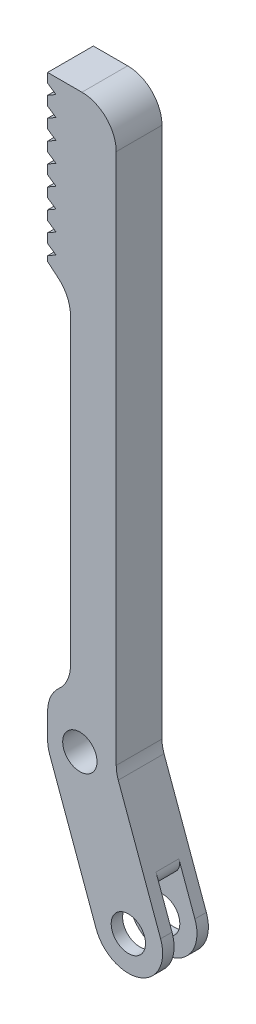
from build123d import *

# Parameters (mm, degrees)
BOSS_EXTRUDE1_DEPTH            = 20
CUT_EXTRUDE1_REACH             = 326.283
SKETCH2_W                      = 10
SKETCH2_H                      = 33.118542384
CUT_EXTRUDE2_DEPTH             = 329.583692554
F_15_0_15_DIAMETER_HOLE1_D     = 15
F_15_0_15_DIAMETER_HOLE1_DEPTH = 5
F_15_0_15_DIAMETER_HOLE2_D     = 15
F_15_0_15_DIAMETER_HOLE3_D     = 15
FILLET1_R                      = 5
FILLET2_R                      = 15
CUT_EXTRUDE3_DEPTH             = 20
SCALE1_SCALE                   = 0.3


with BuildPart() as part:
    # Sketch1 → Boss-Extrude1 (new body)
    with BuildSketch(Plane.XY.offset(20)):
        with BuildLine():
            Line((-35.601097413, 326.0365085), (-35.601097413, 70.746699079))
            Line((-35.601097413, 70.746699079), (-14.395848526, 12.48575659))
            ThreePointArc((-14.395848526, 12.48575659), (4.829842935, 3.520669429), (13.794930097, 22.74636089))
            Line((13.794930097, 22.74636089), (-5.601097413, 76.0365085))
            Line((-5.601097413, 76.0365085), (-5.601097413, 326.0365085))
            Line((-5.601097413, 326.0365085), (-35.601097413, 326.0365085))
        make_face()
    extrude(amount=-BOSS_EXTRUDE1_DEPTH)

    # Sketch2 → Cut-Extrude1 (cut, up to next)
    with BuildSketch(Plane(origin=(19.491769294, 7.094423836, 0), x_dir=(0, 0, -1), z_dir=(0.9396926207859105, 0.3420201433256631, 0)), mode=Mode.PRIVATE) as cut_extrude1_sk1:
        with Locations((-10, 15.602274889)):
            Rectangle(SKETCH2_W, SKETCH2_H)
    cut_extrude1_tool1 = extrude(cut_extrude1_sk1.sketch, amount=-CUT_EXTRUDE1_REACH, mode=Mode.PRIVATE) & part.part
    add(cut_extrude1_tool1.solids().sort_by_distance((14.155477, 21.755766, 10))[0], mode=Mode.SUBTRACT)

    # Sketch3 → Cut-Extrude2 (cut, through all)
    with BuildSketch(Plane(origin=(0, 0, 0), x_dir=(-1, 0, 0), z_dir=(0, 0, -1))):
        with BuildLine():
            Line((35.601097413, 84.169572779), (35.601097413, 254.427504812))
            Line((35.601097413, 254.427504812), (25.601097413, 246.0365085))
            Line((25.601097413, 246.0365085), (25.601097413, 106.530252554))
            ThreePointArc((25.601097413, 106.530252554), (26.908033475, 100.406528198), (30.601097413, 95.349912667))
            ThreePointArc((30.601097413, 95.349912667), (34.29416135, 90.293297136), (35.601097413, 84.169572779))
        make_face()
    extrude(amount=-CUT_EXTRUDE2_DEPTH, mode=Mode.SUBTRACT)

    # Ø15.0 (15) Diameter Hole1
    with Locations(Plane.XY.offset(5)):
        with Locations((-0.300459215, 17.61605874)):
            Hole(F_15_0_15_DIAMETER_HOLE1_D / 2, depth=F_15_0_15_DIAMETER_HOLE1_DEPTH)

    # Ø15.0 (15) Diameter Hole2 (through all)
    with Locations(Plane(origin=(0, 0, 0), x_dir=(-1, 0, 0), z_dir=(0, 0, -1))):
        with Locations((21.505708101, 75.877001229)):
            Hole(F_15_0_15_DIAMETER_HOLE2_D / 2)

    # Ø15.0 (15) Diameter Hole3 (through all)
    with Locations(Plane(origin=(0, 0, 15), x_dir=(-1, 0, 0), z_dir=(0, 0, -1))):
        with Locations((0.300459215, 17.61605874)):
            Hole(F_15_0_15_DIAMETER_HOLE3_D / 2)

    # Fillet1
    fillet1_edges = [part.edges().sort_by_distance(p)[0] for p in [
        (8.491872693, 37.316391362, 10),
    ]]
    fillet(fillet1_edges, radius=FILLET1_R)

    # Fillet2
    fillet2_edges = [part.edges().sort_by_distance(p)[0] for p in [
        (-5.601097413, 326.0365085, 10),
        (-5.601097413, 76.0365085, 10),
        (-35.601097413, 70.746699079, 10),
        (-25.601097413, 246.0365085, 10),
    ]]
    fillet(fillet2_edges, radius=FILLET2_R)

    # Sketch10 → Cut-Extrude3 (cut)
    with BuildSketch(Plane.XY.offset(20)):
        Polygon((-35.601097413, 317.362498495), (-35.601097413, 321.974448946), (-35.601097413, 326.0365085), (-41.358567597, 326.0365085), (-41.358567597, 256.644428456), (-35.601097413, 256.644428456), (-35.601097413, 261.256378908), (-35.601097413, 265.318438462), (-35.601097413, 269.930388913), (-35.601097413, 273.992448467), (-35.601097413, 278.604398919), (-35.601097413, 282.666458473), (-35.601097413, 287.278408924), (-35.601097413, 291.340468478), (-35.601097413, 295.95241893), (-35.601097413, 300.014478484), (-35.601097413, 304.626428935), (-35.601097413, 308.688488489), (-35.601097413, 313.300438941), align=None)
        Polygon((-31.945953564, 310.813956834), (-35.601097413, 313.300438941), (-35.601097413, 308.688488489), align=None)
        Polygon((-31.945953564, 319.487966839), (-35.601097413, 321.974448946), (-35.601097413, 317.362498495), align=None)
        Polygon((-31.945953564, 302.139946828), (-35.601097413, 304.626428935), (-35.601097413, 300.014478484), align=None)
        Polygon((-31.945953564, 293.465936823), (-35.601097413, 295.95241893), (-35.601097413, 291.340468478), align=None)
        Polygon((-31.945953564, 284.791926817), (-35.601097413, 287.278408924), (-35.601097413, 282.666458473), align=None)
        Polygon((-35.601097413, 278.604398919), (-35.601097413, 273.992448467), (-31.945953564, 276.117916812), align=None)
        Polygon((-35.601097413, 269.930388913), (-35.601097413, 265.318438462), (-31.945953564, 267.443906806), align=None)
        Polygon((-35.601097413, 261.256378908), (-35.601097413, 256.644428456), (-31.945953564, 258.769896801), align=None)
    extrude(amount=-CUT_EXTRUDE3_DEPTH, mode=Mode.SUBTRACT)


with BuildPart() as part_1:
    # Scale1: scaled about (0, 0, 0)
    add(part.part.scale(SCALE1_SCALE))


solid = part_1.part
